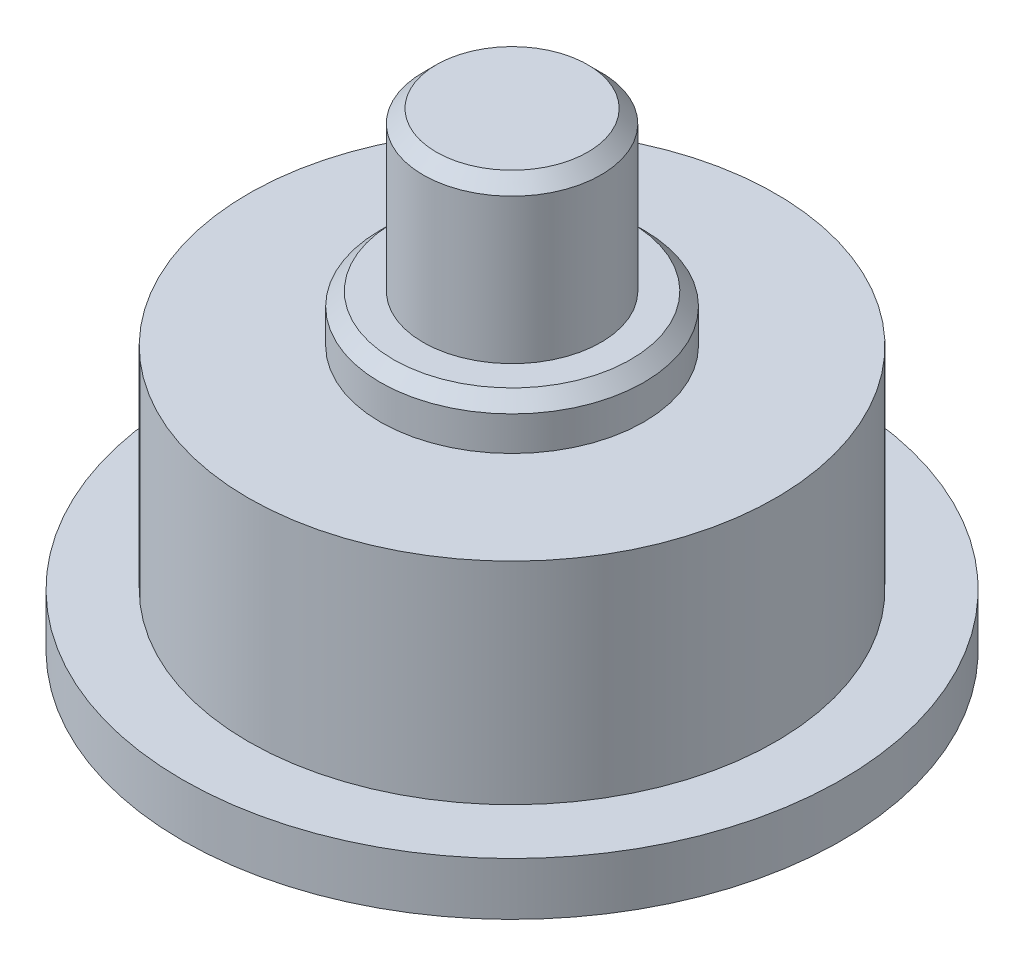
from build123d import *

# Parameters (mm, degrees)
CHAMFER1_SIZE = 0.5


with BuildPart() as part:
    # Sketch1 → Revolve8 (revolve)
    with BuildSketch(Plane.XY, mode=Mode.PRIVATE) as revolve8_sk:
        Polygon((20.861200947, -54.530577635), (24.233987709, -54.530577635), (24.233987709, -72.330577635), (11.733987709, -72.330577635), (11.733987709, -70.330577635), (14.233987709, -70.330577635), (14.233987709, -62.330577635), (19.233987709, -62.330577635), (19.233987709, -60.530577635), (20.861200947, -60.530577635), align=None)
    revolve(revolve8_sk.sketch.rotate(Axis((24.233987709, -52.030577635, 0), (0, -1, 0)), 270), axis=Axis((24.233987709, -52.030577635, 0), (0, -1, 0)))

    # Chamfer1
    chamfer1_edges = [part.edges().sort_by_distance(p)[0] for p in [
        (24.233987709, -54.530577635, -3.372786762),
        (24.233987709, -60.530577635, -5),
    ]]
    chamfer(chamfer1_edges, length=CHAMFER1_SIZE)


solid = part.part
